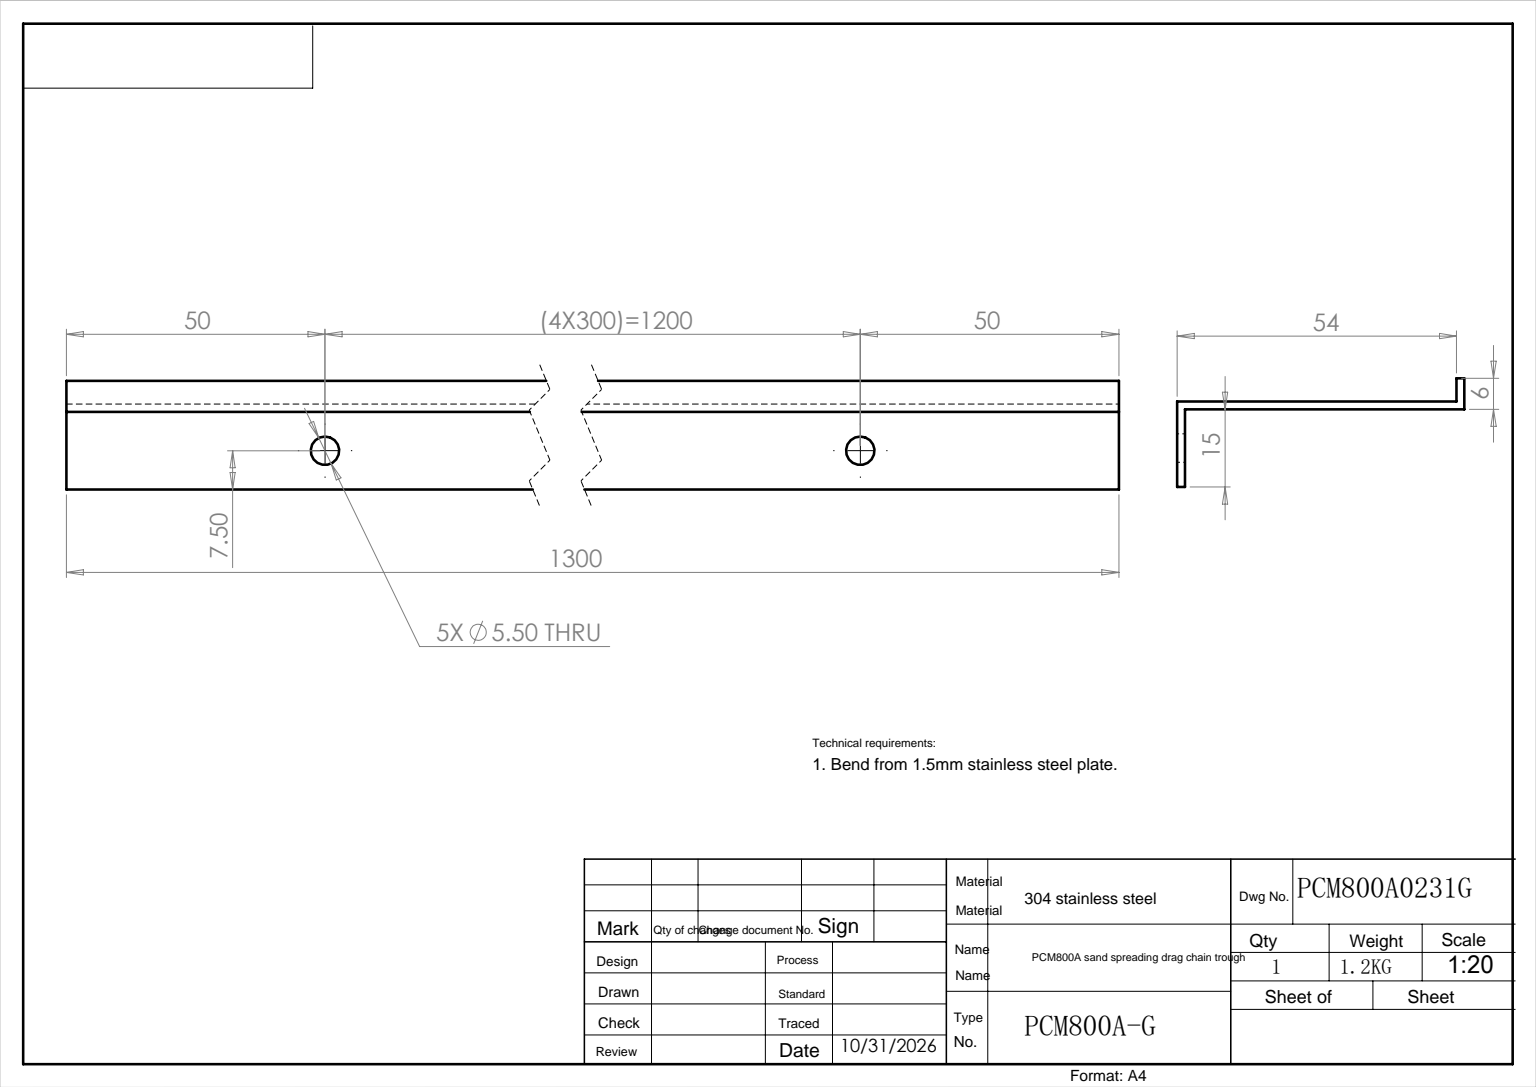
SolidWorks part; units mm, degrees
ref_plane "前视基准面" through (0, 0, 0) normal (0, 0, 1) x (1, 0, 0)
ref_plane "上视基准面" through (0, 0, 0) normal (0, 1, 0) x (1, 0, 0)
ref_plane "右视基准面" through (0, 0, 0) normal (1, 0, 0) x (0, 0, -1)
sketch "草图1" plane through (0, 0, 0) normal (0, 0, 1) x (1, 0, 0)
  line L0 (0, 0) -> (0, -15)
  line L1 (0, 0) -> (54, 0)
  line L2 (54, 0) -> (54, 6)
  dimension "D1" = 6
  dimension "D2" = 15
  dimension "D3" = 54
extrude "拉伸-薄壁1" add sketch "草图1" along normal blind 1300 thin
sketch "草图2" plane through (0, 0, 0) normal (1, 0, 0) x (0, 0, -1)
  line L0 (0, -7.5) -> (-1646.8518, -7.5) construction
  line L2 (0, -15) -> (0, 0) construction
  line L3 (-1300, -15) -> (-1300, 0) construction
  circle A0 centre (-1250, -7.5) radius 2.75
  circle A1 centre (-950, -7.5) radius 2.75
  circle A2 centre (-650, -7.5) radius 2.75
  circle A3 centre (-350, -7.5) radius 2.75
  circle A4 centre (-50, -7.5) radius 2.75
  dimension "D2" = 5.5
  dimension "D1" = 50
  dimension "D3" = 5
extrude "切除-拉伸1" cut sketch "草图2" against normal blind 10
